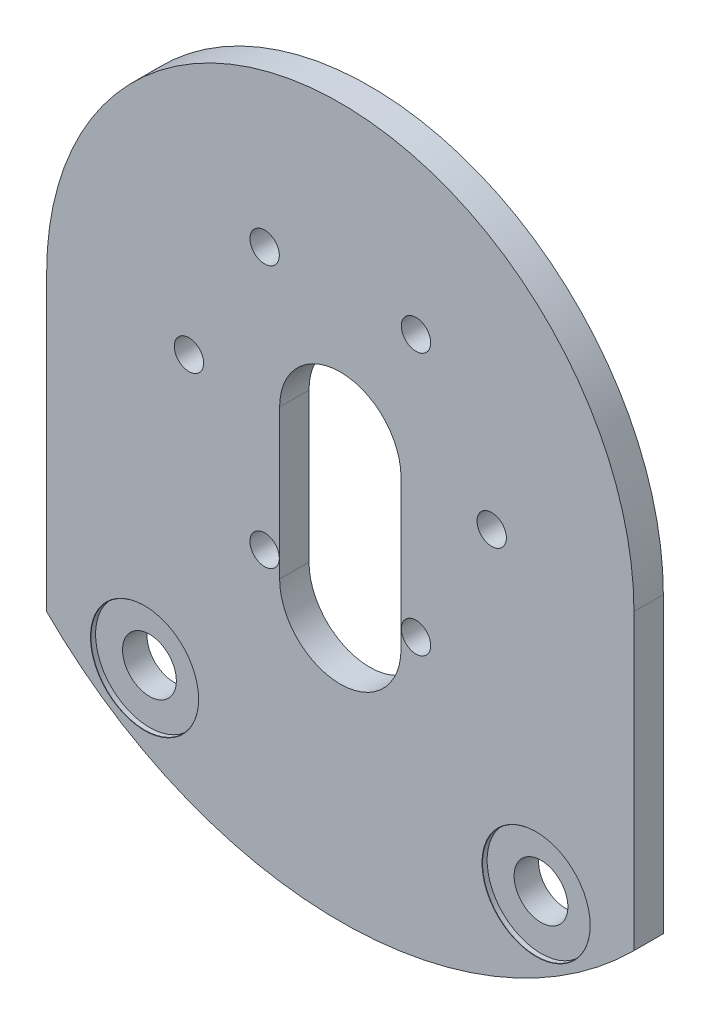
SolidWorks part; units mm, degrees
material "钢"
ref_plane "Front Plane" through (0, 0, 0) normal (0, 0, 1) x (1, 0, 0)
ref_plane "Top Plane" through (0, 0, 0) normal (0, 1, 0) x (1, 0, 0)
ref_plane "Right Plane" through (0, 0, 0) normal (1, 0, 0) x (0, 0, -1)
sketch "Sketch4" plane through (0, 0, 0) normal (0, 0, 1) x (1, 0, 0)
  line L0 (-30, 0) -> (30, 0) construction
  line L1 (30, 0) -> (30, -30)
  line L2 (-30, 0) -> (-30, -30)
  line L4 (0, 0) -> (0, -53.6741) construction
  line L5 (0, 0) -> (0, -15.2188) construction
  line L8 (6.2, 0) -> (6.2, -15.2188)
  line L9 (-6.2, 0) -> (-6.2, -15.2188)
  arc A0 (30, 0) -> (-30, 0) centre (0, 0) ccw
  arc A6 (6.2, 0) -> (-6.2, 0) centre (0, 0) ccw
  arc A7 (-6.2, -15.2188) -> (6.2, -15.2188) centre (0, -15.2188) ccw
  arc A8 (-30, -30) -> (30, -30) centre (0, 0) ccw
  point P8 (0, -7.6094)
  dimension "D1" = 30
  dimension "D4" = 6.2
  dimension "D2" = 30
  dimension "D3" = 30
extrude "Boss-Extrude1" add sketch "Sketch4" along normal blind 3
sketch "Sketch11" plane through (0, 0, 3) normal (0, 0, 1) x (1, 0, 0)
  line L0 (-30, 0) -> (30, 0) construction
  circle A0 centre (0, 0) radius 15.5 construction
  arc A1 (30, 0) -> (-30, 0) centre (0, 0) ccw construction
  circle A2 centre (-15.4638, 0) radius 1.5
  circle A3 centre (0, 0) radius 15.5 construction
  circle A4 centre (-7.7319, 13.392) radius 1.5
  circle A5 centre (0, 0) radius 15.5 construction
  circle A6 centre (7.7319, 13.392) radius 1.5
  circle A7 centre (0, 0) radius 15.5 construction
  circle A8 centre (15.4638, 0) radius 1.5
  circle A9 centre (0, 0) radius 15.5 construction
  circle A10 centre (7.7319, -13.392) radius 1.5
  circle A11 centre (0, 0) radius 15.5 construction
  circle A12 centre (-7.7319, -13.392) radius 1.5
  point P30 (0, 0)
  dimension "D1" = 31
  dimension "D2" = 6
  dimension "D3" = 3
extrude "Cut-Extrude1" cut sketch "Sketch11" against normal blind 3
sketch "Sketch13" plane through (0, 0, 3) normal (0, 0, 1) x (1, 0, 0)
  line L1 (-30, 0) -> (-30, -30) construction
  point P5 (-20, -30)
  point P15 (20, -30)
  dimension "D1" = 10
hole_wizard "CBORE for M5 Hexagon head bolts-Full thread-grade C1" positions "Sketch13" profile "Sketch14" counterbore size "M5" standard "GB" end condition through all
sketch "Sketch14" plane through (20, -30, 3) normal (1, 0, 0) x (0, -1, 0)
  line L0 (0, 0) -> (0, 3)
  line L1 (0, 3) -> (2.75, 3)
  line L3 (2.75, 3) -> (2.75, 0.5)
  line L4 (5.5, 0.5) -> (2.75, 0.5)
  line L5 (5.5, 0.5) -> (5.5, 0.025)
  line L6 (5.5, 0.025) -> (5.525, 0)
  line L7 (5.525, 0) -> (0, 0)
  line L8 (-5.5, 0.025) -> (-5.525, 0) construction
  line L11 (0, -6.35) -> (0, 107.95) construction
  dimension "通孔孔直径" = 5.5
  dimension "通孔孔深度" = 3
  dimension "柱形沉头孔直径" = 11
  dimension "柱形沉头孔深度" = 0.5
  dimension "近端锥形沉头孔直径" = 11.05
  dimension "近端锥形沉头孔角度" = 90
